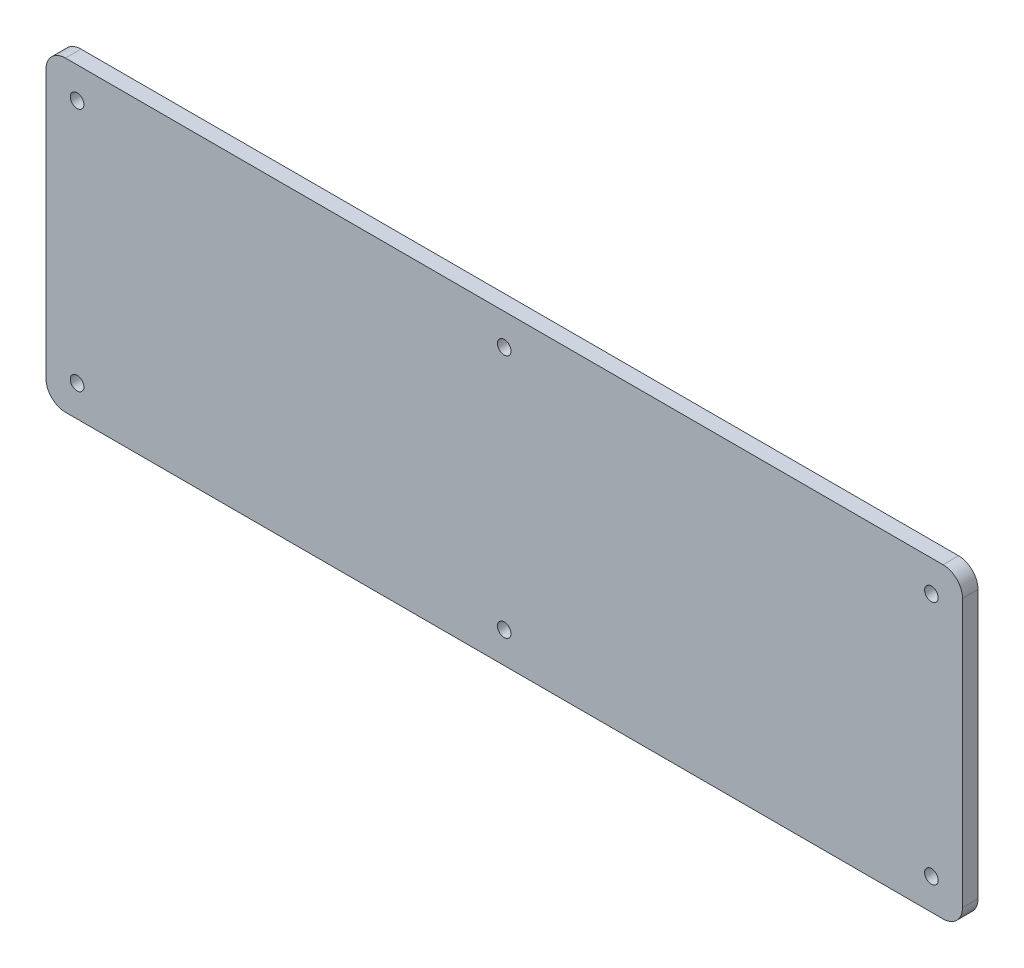
from build123d import *

# Parameters (mm, degrees)
SKETCH1_W           = 236
SKETCH1_H           = 79
BOSS_EXTRUDE1_DEPTH = 4
FILLET1_R           = 5
SKETCH4_R           = 1.75
CUT_EXTRUDE1_DEPTH  = 125.5


with BuildPart() as part:
    # Sketch1 → Boss-Extrude1 (new body)
    with BuildSketch(Plane.XY):
        Rectangle(SKETCH1_W, SKETCH1_H)
    extrude(amount=BOSS_EXTRUDE1_DEPTH)

    # Fillet1
    fillet1_edges = [part.edges().sort_by_distance(p)[0] for p in [
        (-118, 39.5, 2),
        (118, 39.5, 2),
        (118, -39.5, 2),
        (-118, -39.5, 2),
    ]]
    fillet(fillet1_edges, radius=FILLET1_R)

    # Sketch4 → Cut-Extrude1 (cut, through all)
    with BuildSketch(Plane(origin=(0, 0, 0), x_dir=(-1, 0, 0), z_dir=(0, 0, -1))):
        with Locations((-110, 31.5)):
            Circle(SKETCH4_R)
        with Locations((110, 31.5)):
            Circle(SKETCH4_R)
        with Locations((110, -31.5)):
            Circle(SKETCH4_R)
        with Locations((-110, -31.5)):
            Circle(SKETCH4_R)
        with Locations((0, 31.5)):
            Circle(SKETCH4_R)
        with Locations((0, -31.5)):
            Circle(SKETCH4_R)
    extrude(amount=-CUT_EXTRUDE1_DEPTH, mode=Mode.SUBTRACT)


solid = part.part
